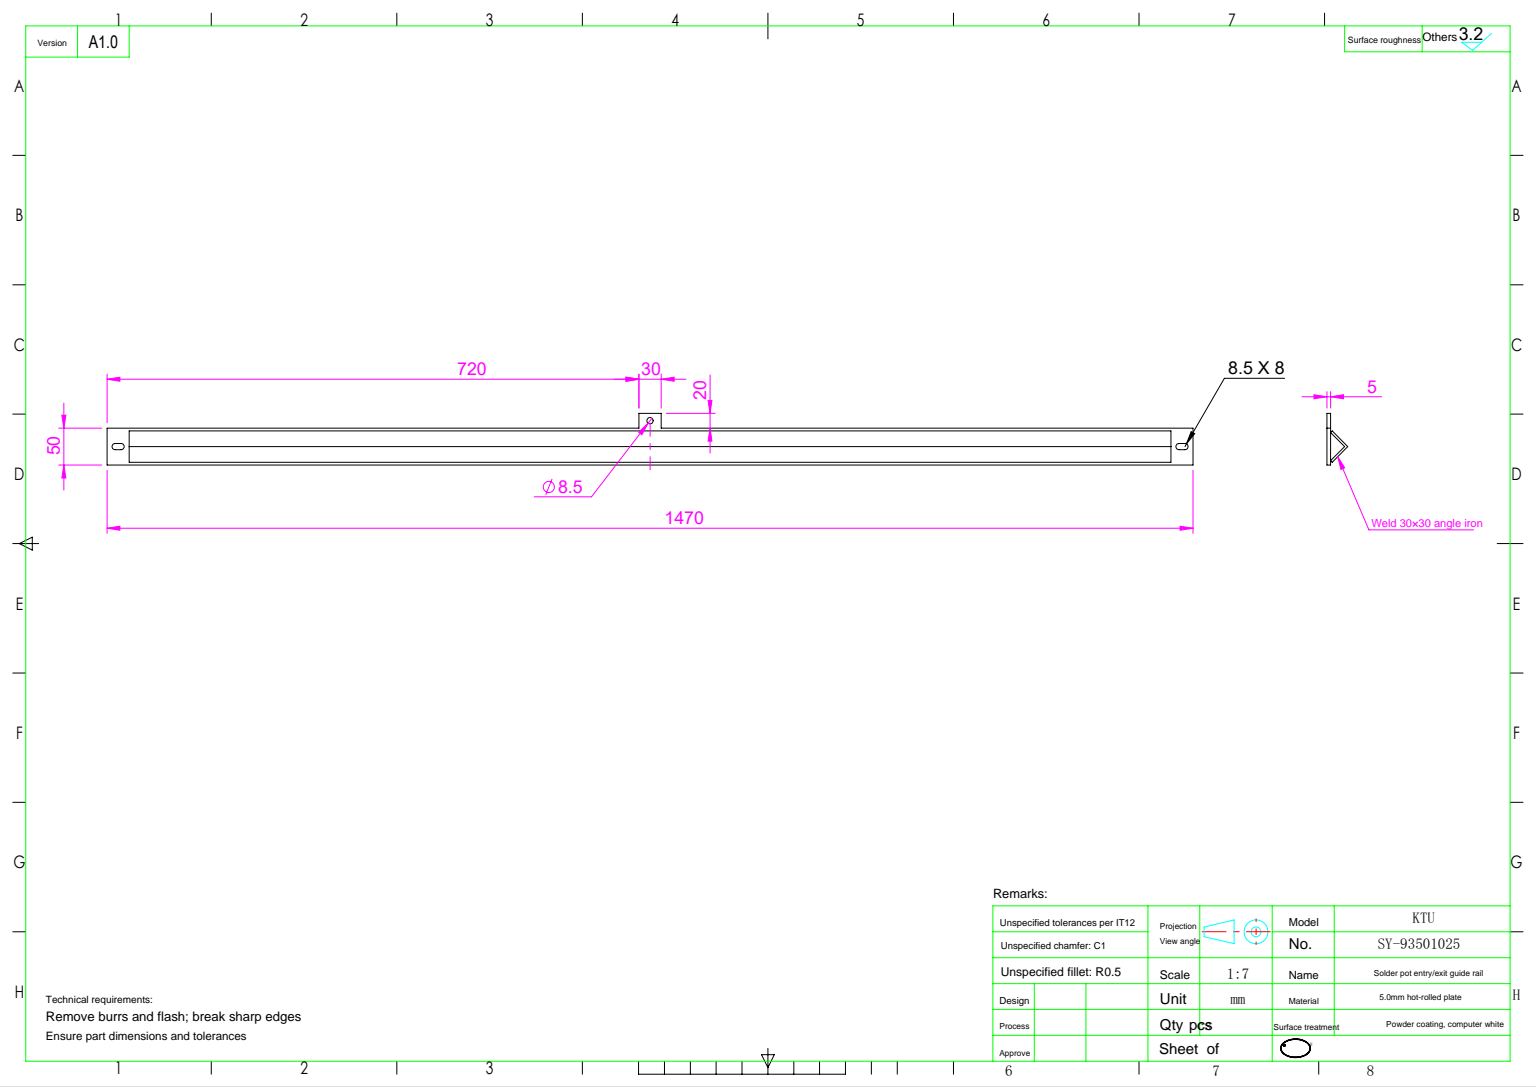
SolidWorks part; units mm, degrees
material "5.0热板"
ref_plane "前视" through (0, 0, 0) normal (0, 0, 1) x (1, 0, 0)
ref_plane "上视" through (0, 0, 0) normal (0, 1, 0) x (1, 0, 0)
ref_plane "右视" through (0, 0, 0) normal (1, 0, 0) x (0, 0, -1)
sketch "草图1" plane through (0, 0, 0) normal (0, 0, 1) x (1, 0, 0)
  line L1 (-735, 25) -> (735, 25)
  line L2 (-735, 25) -> (-735, -25)
  line L3 (-735, -25) -> (735, -25)
  line L4 (735, 25) -> (735, -25)
  line L5 (-735, 25) -> (735, -25) construction
  line L6 (-735, -25) -> (735, 25) construction
  point P0 (0, 0)
  dimension "D1" = 1470
  dimension "D2" = 50
extrude "凸台-拉伸1" add sketch "草图1" along normal mid plane 5
ref_plane "基准面1" through (-705, 0, 0) normal (-1, 0, 0) x (0, 0, 1)
sketch "草图3" plane through (-705, 0, 0) normal (-1, 0, 0) x (0, 0, 1)
  line L0 (2.5, 19.0919) -> (21.5919, 0)
  line L1 (2.5, 25) -> (2.5, -25) construction
  line L2 (21.5919, 0) -> (2.5, -19.0919)
  line L3 (4.6213, 21.2132) -> (25.8345, 0)
  line L4 (25.8345, 0) -> (4.6213, -21.2132)
  line L5 (4.6213, 21.2132) -> (2.5, 19.0919)
  line L6 (2.5, -19.0919) -> (4.6213, -21.2132)
  dimension "D1" = 90
  dimension "D2" = 27
  dimension "D3" = 3
extrude "凸台-拉伸2" add sketch "草图3" against normal blind 1410 separate body
sketch "草图4" plane through (0, 0, 2.5) normal (0, 0, 1) x (1, 0, 0)
  line L0 (716, 0) -> (724, 0) construction
  line L1 (716, 4.25) -> (724, 4.25)
  line L2 (716, -4.25) -> (724, -4.25)
  line L3 (-716, 0) -> (-724, 0) construction
  line L4 (-716, -4.25) -> (-724, -4.25)
  line L5 (-716, 4.25) -> (-724, 4.25)
  line L6 (-735, 25) -> (-735, -25) construction
  line L7 (735, -25) -> (735, 25) construction
  arc A0 (716, 4.25) -> (716, -4.25) centre (716, 0) ccw
  arc A1 (724, -4.25) -> (724, 4.25) centre (724, 0) ccw
  arc A2 (-716, -4.25) -> (-716, 4.25) centre (-716, 0) ccw
  arc A3 (-724, 4.25) -> (-724, -4.25) centre (-724, 0) ccw
  point P2 (720, 0)
  point P9 (-720, 0)
  dimension "D1" = 4.25
  dimension "D2" = 8
  dimension "D3" = 15
  dimension "D4" = 15
extrude "切除-拉伸1" cut sketch "草图4" against normal up to next (5 mm away)
sketch "草图5" plane through (0, 0, 2.5) normal (0, 0, 1) x (1, 0, 0)
  line L0 (735, 25) -> (-735, 25) construction
  line L1 (15, 25) -> (-15, 25)
  line L2 (15, 25) -> (15, 45)
  line L3 (15, 45) -> (-15, 45)
  line L4 (-15, 25) -> (-15, 45)
  dimension "D1" = 30
  dimension "D2" = 15
  dimension "D3" = 20
extrude "凸台-拉伸3" add sketch "草图5" against normal blind 5
sketch "草图6" plane through (0, 0, 2.5) normal (0, 0, 1) x (1, 0, 0)
  line L0 (15, 45) -> (-15, 45) construction
  line L1 (-15, 45) -> (-15, 25) construction
  circle A0 centre (0, 35) radius 4.25
  dimension "D1" = 8.5
  dimension "D2" = 10
  dimension "D3" = 15
extrude "切除-拉伸2" cut sketch "草图6" against normal up to next (5 mm away)
